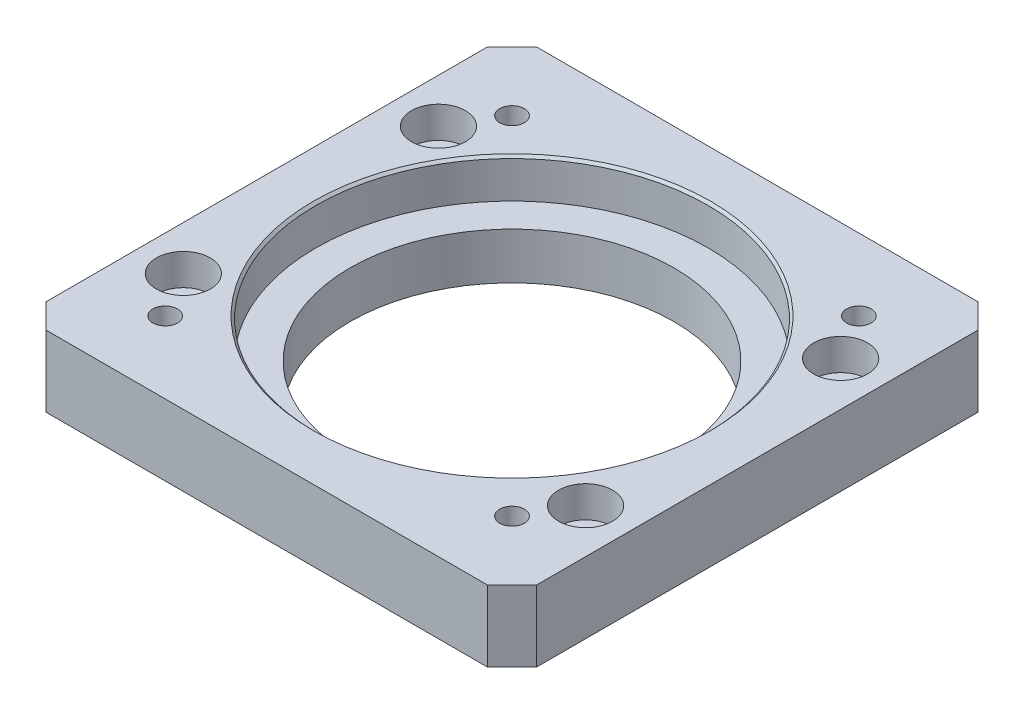
SolidWorks part; units mm, degrees
material "6061Al"
ref_plane "前视基准面" through (0, 0, 0) normal (0, 0, 1) x (1, 0, 0)
ref_plane "上视基准面" through (0, 0, 0) normal (0, 1, 0) x (1, 0, 0)
ref_plane "右视基准面" through (0, 0, 0) normal (1, 0, 0) x (0, 0, -1)
sketch "草图1" plane through (0, 0, 0) normal (0, 1, 0) x (1, 0, 0)
  line L1 (-50, -50) -> (50, -50)
  line L2 (-50, -50) -> (-50, 50)
  line L3 (-50, 50) -> (50, 50)
  line L4 (50, -50) -> (50, 50)
  line L5 (-50, -50) -> (50, 50) construction
  line L6 (-50, 50) -> (50, -50) construction
  point P0 (0, 0)
  dimension "D1" = 100
extrude "凸台-拉伸1" add sketch "草图1" along normal blind 14.5
sketch "草图3" plane through (0, 0, 0) normal (0, -1, 0) x (1, 0, 0)
  circle A0 centre (0, 0) radius 36
  circle A1 centre (0, 0) radius 33
  dimension "D1" = 72
  dimension "D2" = 66
extrude "凸台-拉伸2" add sketch "草图3" along normal blind 3
sketch "草图4" plane through (0, 0, 0) normal (0, -1, 0) x (1, 0, 0)
  circle A1 centre (0, 0) radius 33
  circle A3 centre (0, 0) radius 33
  dimension "D1" = 0
extrude "切除-拉伸1" cut sketch "草图4" against normal through all
sketch "草图5" plane through (0, 14.5, 0) normal (0, 1, 0) x (1, 0, 0)
  circle A0 centre (0, 0) radius 55
  dimension "D1" = 110
extrude "切除-拉伸2" [suppressed] cut sketch "草图5" against normal blind 5
chamfer "倒角1" distance 5 angle 45 4 edges at (-50, 7.25, 50) (50, 7.25, 50) (50, 7.25, -50) (-50, 7.25, -50)
chamfer "倒角2" distance 0.5 angle 45 1 edges at (0, -3, -36)
sketch "草图10" plane through (0, 14.5, 0) normal (0, 1, 0) x (1, 0, 0)
  circle A0 centre (0, 0) radius 40
  dimension "D1" = 80
extrude "切除-拉伸3" cut sketch "草图10" against normal blind 8
sketch "草图12" plane through (0, 14.5, 0) normal (0, 1, 0) x (1, 0, 0)
  line L1 (-50, -50) -> (50, -50)
  line L2 (-50, -50) -> (-50, 50)
  line L3 (-50, 50) -> (50, 50)
  line L4 (50, -50) -> (50, 50)
  line L5 (-50, -50) -> (50, 50) construction
  line L6 (-50, 50) -> (50, -50) construction
  point P0 (0, 0)
  dimension "D1" = 100
extrude "切除-拉伸4" [suppressed] cut sketch "草图12" against normal blind 3
hole_wizard "M6 螺纹孔1" positions "草图13" profile "草图14" tap size "M6" standard "ISO"
sketch "草图13" plane through (0, 14.5, 0) normal (0, 1, 0) x (1, 0, 0)
  line L1 (-35.355, -35.355) -> (35.355, -35.355)
  line L2 (-35.355, -35.355) -> (-35.355, 35.355)
  line L3 (-35.355, 35.355) -> (35.355, 35.355)
  line L4 (35.355, -35.355) -> (35.355, 35.355)
  line L5 (-35.355, -35.355) -> (35.355, 35.355) construction
  line L6 (-35.355, 35.355) -> (35.355, -35.355) construction
  point P0 (-35.355, 35.355)
  point P3 (0, 0)
  point P4 (35.355, 35.355)
  point P7 (-35.355, -35.355)
  point P9 (35.355, -35.355)
  dimension "D1" = 70.71
sketch "草图14" plane through (-35.355, 14.5, -35.355) normal (1, 0, 0) x (0, 0, 1)
  line L0 (0, 0) -> (0, 16.5022)
  line L1 (0, 16.5022) -> (2.5, 15)
  line L2 (2.5, 15) -> (2.5, 0)
  line L5 (2.5, 0) -> (0, 0)
  line L10 (0, 16.5022) -> (-2.5, 15) construction
  line L11 (0, -6.35) -> (0, 107.95) construction
  dimension "螺纹孔钻头直径" = 5
  dimension "螺纹孔钻头深度" = 15
  dimension "导头角度" = 118
cosmetic thread "孔螺蚊线5" parameters "D1"=12, "D2"=6
cosmetic thread "孔螺蚊线6" parameters "D1"=12, "D2"=6
cosmetic thread "孔螺蚊线7" parameters "D1"=12, "D2"=6
cosmetic thread "孔螺蚊线8" parameters "D1"=12, "D2"=6
hole_wizard "M6 六角凹头螺钉的柱形沉头孔1" positions "草图6" profile "草图7" counterbore size "M6" standard "ISO"
sketch "草图6" plane through (0, 22, 0) normal (0, 1, 0) x (1, 0, 0)
  line L8 (0, -42.4264) -> (42.4264, 0)
  line L9 (0, -42.4264) -> (-42.4264, 0)
  line L10 (-42.4264, 0) -> (0, 42.4264)
  line L11 (42.4264, 0) -> (0, 42.4264)
  line L12 (0, -42.4264) -> (0, 42.4264) construction
  line L13 (-42.4264, 0) -> (42.4264, 0) construction
  point P0 (0, 42.4264)
  point P3 (-42.4264, 0)
  point P6 (0, -42.4264)
  point P9 (42.4264, 0)
  point P13 (0, 0)
  point P56 (0, 0)
  dimension "D1" = 60
sketch "草图7" plane through (0, 22, -42.4264) normal (1, 0, 0) x (0, 0, 1)
  line L0 (0, 0) -> (0, 25)
  line L1 (0, 25) -> (3.3, 25)
  line L3 (3.3, 25) -> (3.3, 14.8)
  line L4 (3.3, 14.8) -> (5.5, 14.8)
  line L5 (5.5, 14.8) -> (5.5, 0)
  line L7 (5.5, 0) -> (0, 0)
  line L11 (0, -6.35) -> (0, 107.95) construction
  dimension "通孔孔直径" = 6.6
  dimension "通孔孔深度" = 25
  dimension "柱形沉头孔直径" = 11
  dimension "柱形沉头孔深度" = 14.8
fillet "圆角1" [suppressed] radius 5
hole_wizard "M8 螺纹孔1" positions "草图8" profile "草图9" tap size "M8" standard "ISO"
sketch "草图8" plane through (0, 25, 0) normal (0, 1, 0) x (1, 0, 0)
  line L1 (-51.265, -51.265) -> (51.265, -51.265)
  line L2 (-51.265, -51.265) -> (-51.265, 51.265)
  line L3 (-51.265, 51.265) -> (51.265, 51.265)
  line L4 (51.265, -51.265) -> (51.265, 51.265)
  line L5 (-51.265, -51.265) -> (51.265, 51.265) construction
  line L6 (-51.265, 51.265) -> (51.265, -51.265) construction
  point P0 (51.265, 51.265)
  point P3 (51.265, -51.265)
  point P6 (-51.265, -51.265)
  point P9 (-51.265, 51.265)
  point P13 (0, 0)
  dimension "D1" = 102.53
sketch "草图9" plane through (51.265, 25, -51.265) normal (1, 0, 0) x (0, 0, 1)
  line L0 (0, 0) -> (0, 28)
  line L1 (0, 28) -> (3.4, 28)
  line L2 (3.4, 28) -> (3.4, 0)
  line L5 (3.4, 0) -> (0, 0)
  line L11 (0, -6.35) -> (0, 107.95) construction
  dimension "通孔螺纹孔钻头直径" = 6.8
  dimension "通孔螺纹孔钻头深度" = 28
cosmetic thread "孔螺蚊线1" [suppressed] parameters "D2"=8
cosmetic thread "孔螺蚊线2" [suppressed] parameters "D2"=8
cosmetic thread "孔螺蚊线3" [suppressed] parameters "D2"=8
cosmetic thread "孔螺蚊线4" [suppressed] parameters "D2"=8
sketch "草图15" plane through (0, -3, 0) normal (0, -1, 0) x (1, 0, 0)
  circle A0 centre (0, 0) radius 36.25
  dimension "D1" = 72.5
extrude "切除-拉伸5" [suppressed] cut sketch "草图15" against normal through all
hole_wizard "M6 六角凹头螺钉的柱形沉头孔2" positions "草图16" profile "草图17" counterbore size "M6" standard "ISO" end condition through all
sketch "草图16" plane through (0, 14.5, 0) normal (0, 1, 0) x (1, 0, 0)
  line L1 (41, -26) -> (-41, -26)
  line L2 (41, -26) -> (41, 26)
  line L3 (41, 26) -> (-41, 26)
  line L4 (-41, -26) -> (-41, 26)
  line L5 (41, -26) -> (-41, 26) construction
  line L6 (41, 26) -> (-41, -26) construction
  line L8 (50, -45) -> (50, 45) construction
  point P0 (-41, 26)
  point P3 (0, 0)
  point P7 (41, -26)
  point P8 (41, 26)
  point P9 (-41, -26)
  dimension "D1" = 52
  dimension "9" = 9
sketch "草图17" plane through (-41, 14.5, -26) normal (1, 0, 0) x (0, 0, 1)
  line L0 (0, 0) -> (0, 17.5)
  line L1 (0, 17.5) -> (3.3, 17.5)
  line L3 (3.3, 17.5) -> (3.3, 6.4)
  line L4 (3.3, 6.4) -> (5.5, 6.4)
  line L5 (5.5, 6.4) -> (5.5, 0)
  line L7 (5.5, 0) -> (0, 0)
  line L11 (0, -6.35) -> (0, 107.95) construction
  dimension "通孔孔直径" = 6.6
  dimension "通孔孔深度" = 17.5
  dimension "柱形沉头孔直径" = 11
  dimension "柱形沉头孔深度" = 6.4
chamfer "倒角3" distance 0.5 angle 45 1 edges at (0, 14.5, 40)
